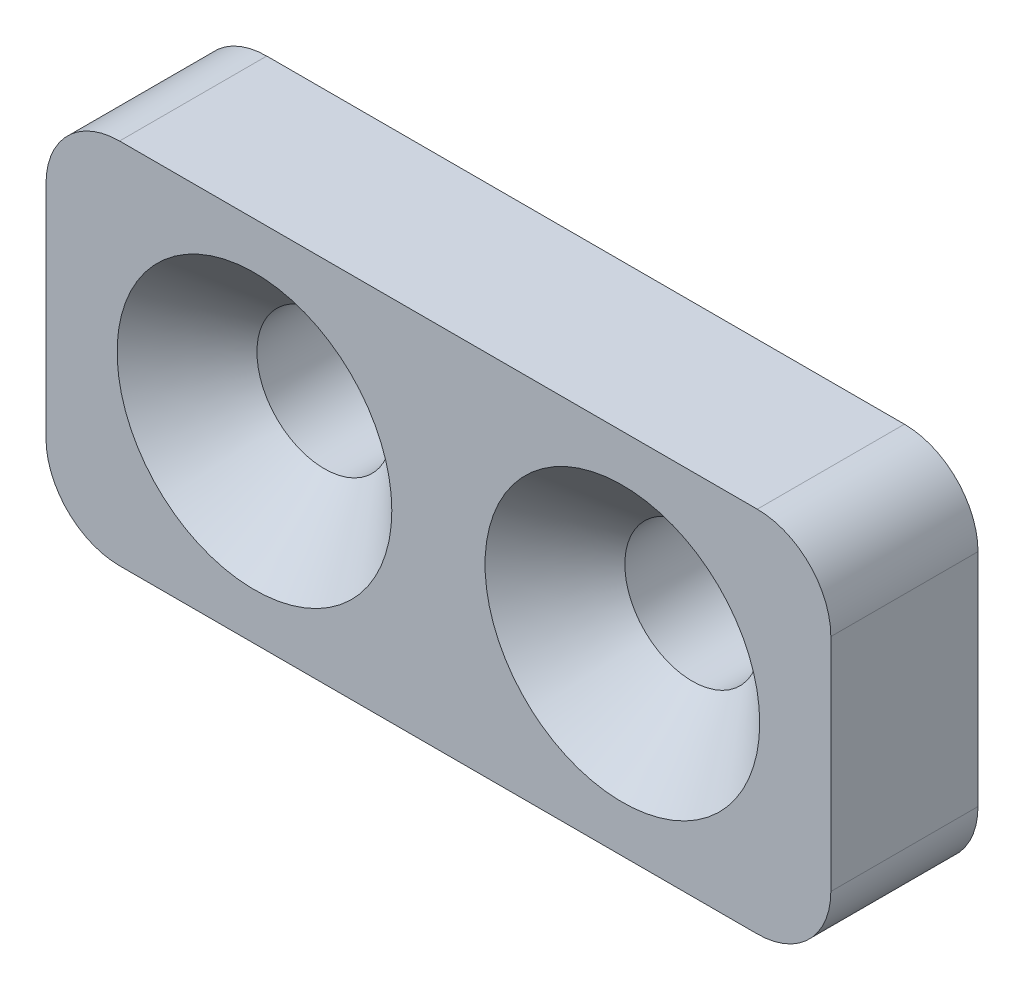
from build123d import *

# Parameters (mm, degrees)
SKETCH1_W                                            = 32
SKETCH1_H                                            = 15
BOSS_EXTRUDE1_DEPTH                                  = 6
CSK_FOR_M5_SLOTTED_RAISED_CTSK_HEAD_WOOD_D           = 5.5
CSK_FOR_M5_SLOTTED_RAISED_CTSK_HEAD_WOOD_DEPTH       = 12.4
CSK_FOR_M5_SLOTTED_RAISED_CTSK_HEAD_WOOD_CSINK_D     = 11.2
CSK_FOR_M5_SLOTTED_RAISED_CTSK_HEAD_WOOD_CSINK_ANGLE = 90
CSK_FOR_M5_SLOTTED_RAISED_CTSK_HEAD_WOOD_TIP         = 1.652366702
FILLET1_R                                            = 3


with BuildPart() as part:
    # Sketch1 → Boss-Extrude1 (new body)
    with BuildSketch(Plane.XY):
        Rectangle(SKETCH1_W, SKETCH1_H)
    extrude(amount=BOSS_EXTRUDE1_DEPTH)

    # CSK for M5 Slotted raised CTSK head wood screws1
    with Locations(Plane.XY.offset(6)):
        with Locations((7.5, 0), (60, 0), (-60, 0), (-7.5, 0)):
            CounterSinkHole(CSK_FOR_M5_SLOTTED_RAISED_CTSK_HEAD_WOOD_D / 2, CSK_FOR_M5_SLOTTED_RAISED_CTSK_HEAD_WOOD_CSINK_D / 2, depth=CSK_FOR_M5_SLOTTED_RAISED_CTSK_HEAD_WOOD_DEPTH, counter_sink_angle=CSK_FOR_M5_SLOTTED_RAISED_CTSK_HEAD_WOOD_CSINK_ANGLE)
            with Locations((0, 0, -(CSK_FOR_M5_SLOTTED_RAISED_CTSK_HEAD_WOOD_DEPTH + CSK_FOR_M5_SLOTTED_RAISED_CTSK_HEAD_WOOD_TIP / 2))):  # 118° drill point
                Cone(0, CSK_FOR_M5_SLOTTED_RAISED_CTSK_HEAD_WOOD_D / 2, CSK_FOR_M5_SLOTTED_RAISED_CTSK_HEAD_WOOD_TIP, mode=Mode.SUBTRACT)

    # Fillet1
    fillet1_edges = [part.edges().sort_by_distance(p)[0] for p in [
        (16, -7.5, 3),
        (-16, -7.5, 3),
        (-16, 7.5, 3),
        (16, 7.5, 3),
    ]]
    fillet(fillet1_edges, radius=FILLET1_R)


solid = part.part
